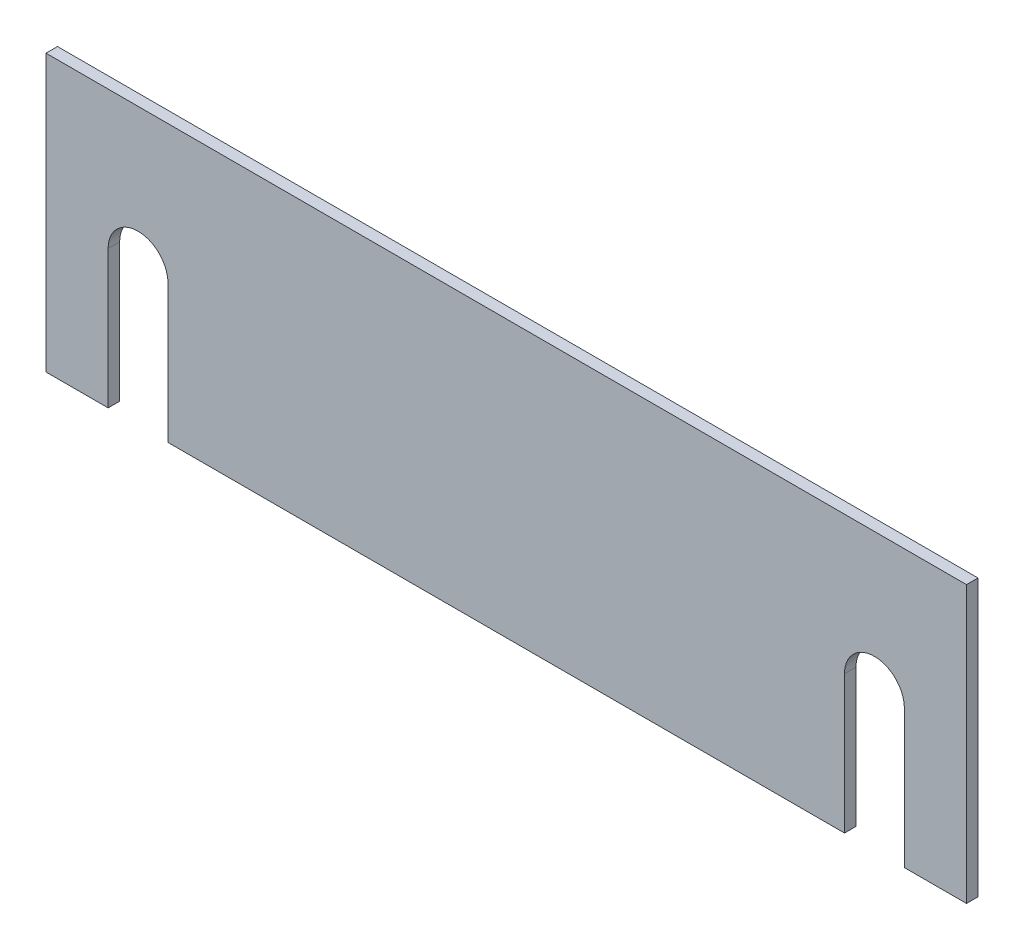
from build123d import *

# Parameters (mm, degrees)
SKETCH1_W           = 400
SKETCH1_H           = 120
BOSS_EXTRUDE1_DEPTH = 5
CUT_EXTRUDE1_DEPTH  = 209.865985742


with BuildPart() as part:
    # Sketch1 → Boss-Extrude1 (new body)
    with BuildSketch(Plane.XY):
        Rectangle(SKETCH1_W, SKETCH1_H)
    extrude(amount=BOSS_EXTRUDE1_DEPTH)

    # Sketch2 → Cut-Extrude1 (cut, through all)
    with BuildSketch(Plane.XY.offset(5)):
        with BuildLine():
            Line((-147, 0), (-147, -96.926835552))
            ThreePointArc((-147, -96.926835552), (-160, -109.926835552), (-173, -96.926835552))
            Line((-173, -96.926835552), (-173, 0))
            ThreePointArc((-173, 0), (-160, 13), (-147, 0))
        make_face()
        with BuildLine():
            Line((147, 0), (147, -96.926835552))
            ThreePointArc((147, -96.926835552), (160, -109.926835552), (173, -96.926835552))
            Line((173, -96.926835552), (173, 0))
            ThreePointArc((173, 0), (160, 13), (147, 0))
        make_face()
    extrude(amount=-CUT_EXTRUDE1_DEPTH, mode=Mode.SUBTRACT)


solid = part.part
